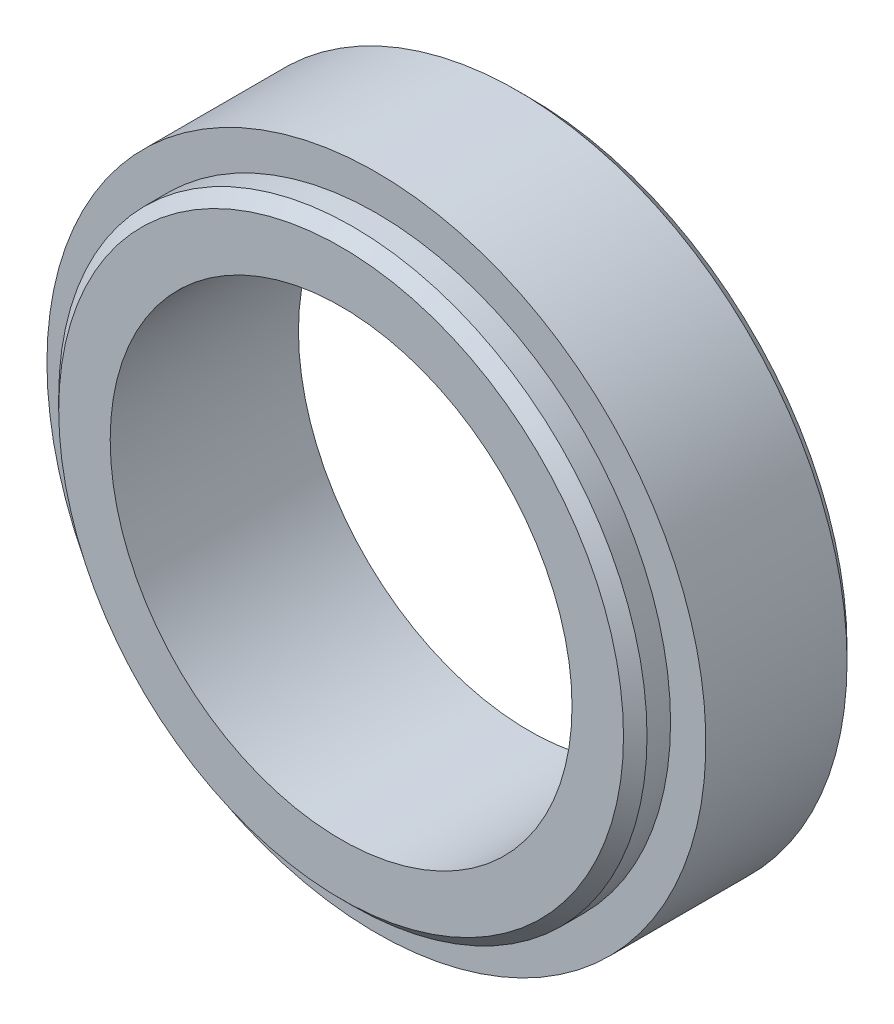
from build123d import *

# Parameters (mm, degrees)
SKETCH1_R           = 28
BOSS_EXTRUDE1_DEPTH = 13
SKETCH2_R           = 25
BOSS_EXTRUDE2_DEPTH = 3
CHAMFER1_SIZE       = 1


with BuildPart() as part:
    # Sketch1 → Boss-Extrude1 (new body)
    with BuildSketch(Plane.XY):
        with Locations(Location((0, 0, 0), (0, 0, 180))):
            Circle(SKETCH1_R)
    extrude(amount=BOSS_EXTRUDE1_DEPTH)

    # Sketch2 → Boss-Extrude2 (add)
    with BuildSketch(Plane.XY.offset(13)):
        Circle(SKETCH2_R)
    extrude(amount=BOSS_EXTRUDE2_DEPTH)

    # Chamfer1
    chamfer1_edges = [part.edges().sort_by_distance(p)[0] for p in [
        (28, 0, 0),
        (-25, 0, 16),
    ]]
    chamfer(chamfer1_edges, length=CHAMFER1_SIZE)

    # Sketch4 → G1-1/4 Tapped Hole1 (revolve, cut)
    with BuildSketch(Plane(origin=(0, 0, 16), x_dir=(0, -1, 0), z_dir=(1, 0, 0))):
        Polygon((0, 0), (0, 102.538889648), (19.625, 90.747), (19.625, 0), align=None)
    revolve(axis=Axis((0, 0, 22.35), (0, 0, -1)), mode=Mode.SUBTRACT)


solid = part.part
